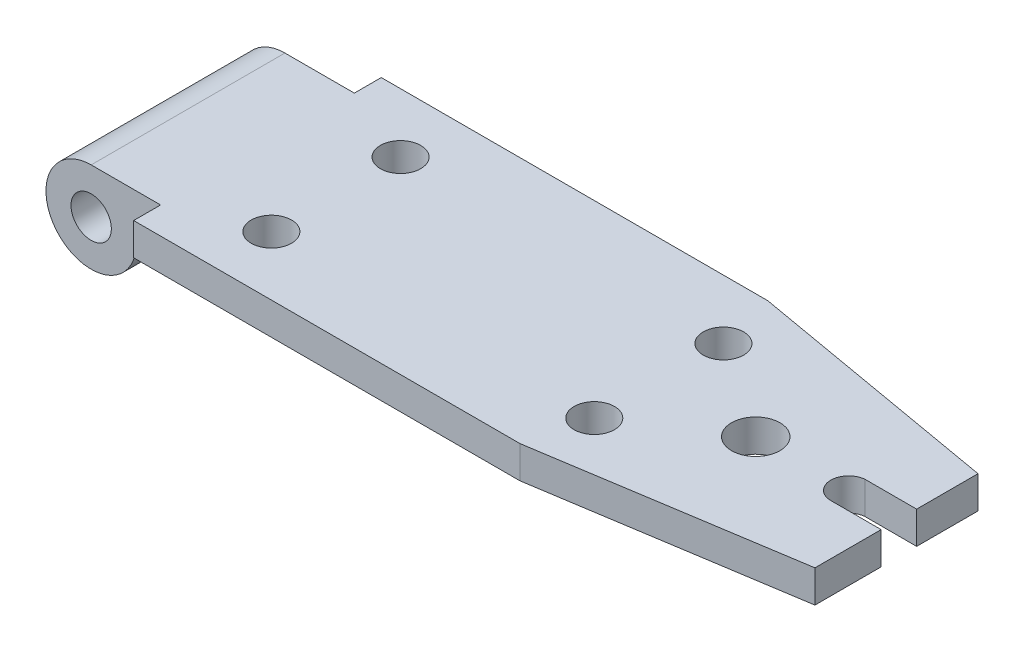
SolidWorks part; units mm, degrees
ref_plane "Front Plane" through (0, 0, 0) normal (0, 0, 1) x (1, 0, 0)
ref_plane "Top Plane" through (0, 0, 0) normal (0, 1, 0) x (1, 0, 0)
ref_plane "Right Plane" through (0, 0, 0) normal (1, 0, 0) x (0, 0, -1)
sketch "Sketch1" plane through (0, 0, 0) normal (0, 1, 0) x (1, 0, 0)
  line L0 (-385.3389, 0) -> (281.505, 0) construction
  line L1 (-156.7667, -76.6872) -> (82.5749, -76.6872)
  line L2 (-171.7667, -60) -> (-171.7667, 60)
  line L3 (-156.7667, 76.6872) -> (82.5749, 76.6872)
  line L4 (82.5749, 76.6872) -> (240.5112, 49)
  line L5 (82.5749, 76.6872) -> (82.5749, -76.6872)
  line L6 (240.5112, 49) -> (240.5112, 11)
  line L7 (-171.7667, 60) -> (-156.7667, 60)
  line L8 (-171.7667, 60) -> (-171.7667, -60)
  line L9 (-156.7667, 60) -> (-156.7667, 76.6872)
  line L10 (-156.7667, -60) -> (-156.7667, -76.6872)
  line L11 (82.5749, -76.6872) -> (240.5112, -51.9911)
  line L12 (240.5112, 11) -> (208.5112, 11)
  line L13 (240.5112, -11) -> (208.5112, -11)
  line L14 (240.5112, -11) -> (240.5112, -51.9911)
  line L15 (-171.7667, -60) -> (-156.7667, -60)
  circle A0 centre (-108.1504, 40) radius 12.5
  circle A1 centre (-108.1504, -40) radius 12.5
  circle A2 centre (91.8496, 40) radius 12.5
  circle A3 centre (91.8496, -40) radius 12.5
  circle A4 centre (151.8496, 0) radius 15
  arc A5 (208.5112, 11) -> (208.5112, -11) centre (209.4135, 0) ccw
  point P0 (0, 0)
  point P2 (0, 0)
  point P25 (247.7352, 0)
  dimension "D2" = 49
  dimension "D6" = 60
  dimension "D7" = 25
  dimension "D8" = 25
  dimension "D9" = 25
  dimension "D10" = 25
  dimension "D11" = 30
  dimension "D14" = 22
  dimension "D3" = 32
  dimension "D4" = 40
  dimension "D5" = 60
  dimension "D12" = 80
  dimension "D13" = 15
  dimension "D15" = 200
extrude "Boss-Extrude1" add sketch "Sketch1" along normal blind 20
sketch "Sketch2" plane through (0, 0, 0) normal (0, 0, 1) x (1, 0, 0)
  line L0 (-171.7667, 20) -> (-199.7667, 20) construction
  line L1 (-199.7667, 20) -> (-171.7667, 20)
  line L2 (-156.7667, 20) -> (82.5749, 20) construction
  line L3 (-171.7667, 20) -> (-171.7667, -8)
  arc A0 (-199.7667, 20) -> (-171.7667, -8) centre (-199.7667, -8) ccw
  circle A1 centre (-199.7667, -8) radius 12.5
  arc A2 (-199.7667, 20) -> (-171.7667, -8) centre (-199.7667, -8) ccw
  dimension "D1" = 56
  dimension "D3" = 25
  dimension "D2" = 28
extrude "Boss-Extrude3" add sketch "Sketch2" along normal mid plane 120 contours L1 A0 L3 A1
